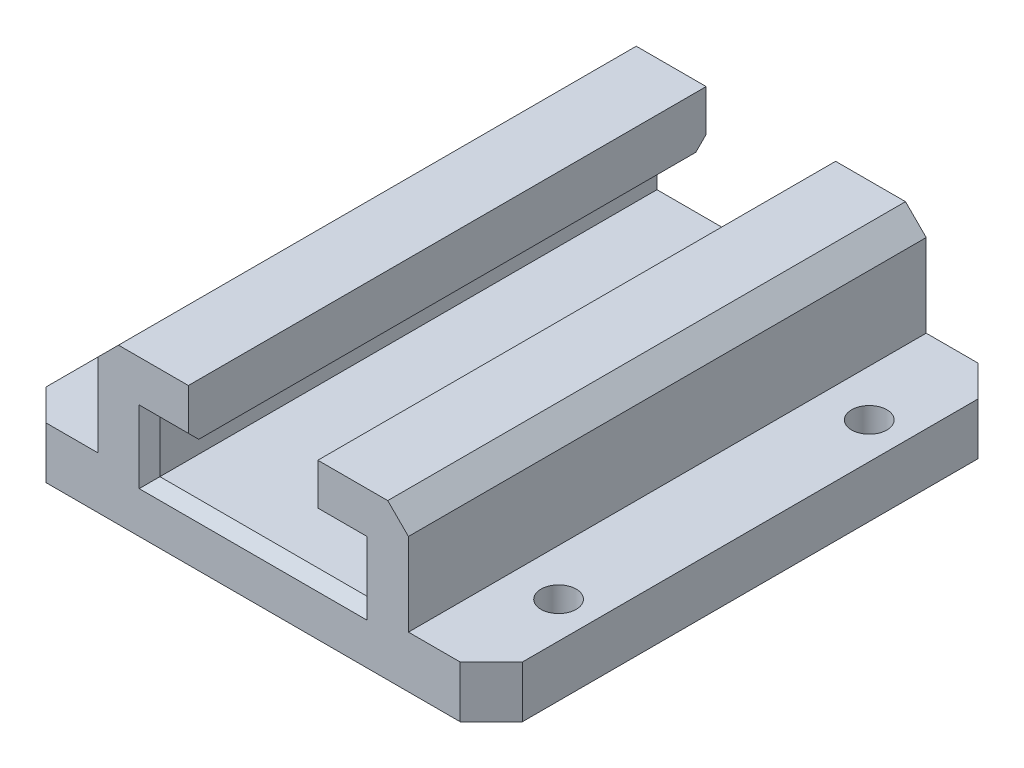
SolidWorks part; units mm, degrees
ref_plane "前视基准面" through (0, 0, 0) normal (0, 0, 1) x (1, 0, 0)
ref_plane "上视基准面" through (0, 0, 0) normal (0, 1, 0) x (1, 0, 0)
ref_plane "右视基准面" through (0, 0, 0) normal (1, 0, 0) x (0, 0, -1)
sketch "草图1" plane through (0, 0, 0) normal (0, 0, 1) x (1, 0, 0)
  line L0 (0, 0) -> (0, 28.1365) construction
  line L1 (15, 0) -> (-15, 0)
  line L2 (-15, 0) -> (-15, 15)
  line L3 (-15, 15) -> (-6.25, 15)
  line L4 (-6.25, 15) -> (-6.25, 10)
  line L5 (-6.25, 10) -> (-10, 10)
  line L6 (-10, 10) -> (-10, 5)
  line L7 (-10, 5) -> (10, 5)
  line L8 (10, 10) -> (10, 5)
  line L9 (6.25, 10) -> (10, 10)
  line L10 (6.25, 15) -> (6.25, 10)
  line L11 (15, 15) -> (6.25, 15)
  line L12 (15, 0) -> (15, 15)
  point P12 (0, 5)
  dimension "D1" = 20
  dimension "D2" = 5
  dimension "D3" = 15
  dimension "D4" = 5
  dimension "D5" = 30
  dimension "D6" = 12.5
extrude "凸台-拉伸1" add sketch "草图1" along normal blind 50
sketch "草图3" plane through (0, 0, 50) normal (0, 0, 1) x (1, 0, 0)
  line L0 (0, 0) -> (0, 23.4202) construction
  line L1 (-15, 0) -> (-23, 0)
  line L2 (-15, 0) -> (-15, 5)
  line L3 (-15, 5) -> (-23, 5)
  line L4 (-23, 0) -> (-23, 5)
  line L5 (23, 0) -> (23, 5)
  line L6 (15, 5) -> (23, 5)
  line L7 (15, 0) -> (15, 5)
  line L8 (15, 0) -> (23, 0)
  dimension "D1" = 8
  dimension "D2" = 5
extrude "凸台-拉伸2" add sketch "草图3" against normal up to surface (50 mm away) up to face at (0, 9.1667, 0)
chamfer "倒角1" distance 1 angle 45 5 edges at (8.125, 10, 50) (10, 7.5, 50) (-8.125, 10, 50) (-10, 7.5, 50) (0, 5, 50)
chamfer "倒角2" distance 1 angle 45 5 edges at (8.125, 10, 0) (-8.125, 10, 0) (-10, 7.5, 0) (0, 5, 0) (10, 7.5, 0)
chamfer "倒角3" distance 3 angle 45 4 edges at (-23, 2.5, 0) (-23, 2.5, 50) (23, 2.5, 0) (23, 2.5, 50)
sketch "草图6" plane through (0, 5, 0) normal (0, 1, 0) x (1, 0, 0)
  line L0 (0, 0) -> (0, -55.7829) construction
  line L2 (6.25, -25) -> (40.2521, -25) construction
  line L3 (6.25, -50) -> (6.25, 0) construction
  point P0 (-19.5, -10)
  point P2 (-19.5, -40)
  point P10 (19.5, -40)
  point P11 (19.5, -10)
  dimension "D1" = 39
  dimension "D2" = 30
hole_wizard "M3 间隙孔1" positions "草图6" profile "草图5" hole size "M3" standard "GB" end condition through all
sketch "草图5" plane through (-19.5, 5, 10) normal (1, 0, 0) x (0, 0, 1)
  line L0 (0, 0) -> (0, 5)
  line L1 (0, 5) -> (1.7, 5)
  line L2 (1.7, 5) -> (1.7, 0)
  line L5 (1.7, 0) -> (0, 0)
  line L11 (0, -6.35) -> (0, 107.95) construction
  dimension "通孔孔直径" = 3.4
  dimension "通孔孔深度" = 5
chamfer "倒角4" distance 2 angle 45 2 edges at (-15, 15, 25) (15, 15, 25)
